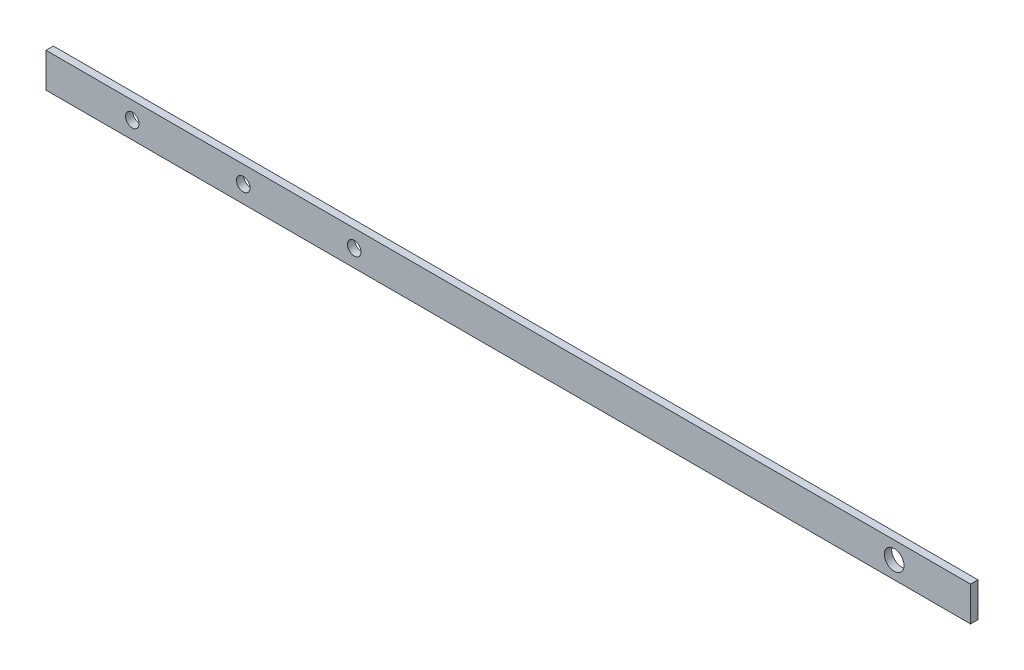
from build123d import *

# Parameters (mm, degrees)
SKETCH_1_W          = 375
SKETCH_1_H          = 14
SKETCH_1_R          = 2.75
EXTRUDE_1_DEPTH     = 1.5
SKETCH_2_R          = 4
CUT_EXTRUDE_1_DEPTH = 3


with BuildPart() as part:
    # 草图1 → 凸台-拉伸1 (new, symmetric)
    with BuildSketch(Plane.XY):
        Rectangle(SKETCH_1_W, SKETCH_1_H)
        with Locations((-152.5, 0)):
            Circle(SKETCH_1_R, mode=Mode.SUBTRACT)
        with Locations((-107.5, 0)):
            Circle(SKETCH_1_R, mode=Mode.SUBTRACT)
        with Locations((-62.5, 0)):
            Circle(SKETCH_1_R, mode=Mode.SUBTRACT)
    extrude(amount=EXTRUDE_1_DEPTH, both=True)

    # 草图2 → 切除-拉伸1 (cut)
    with BuildSketch(Plane.XY.offset(1.5)):
        with Locations((156.5, 0)):
            Circle(SKETCH_2_R)
    extrude(amount=-CUT_EXTRUDE_1_DEPTH, mode=Mode.SUBTRACT)


solid = part.part
